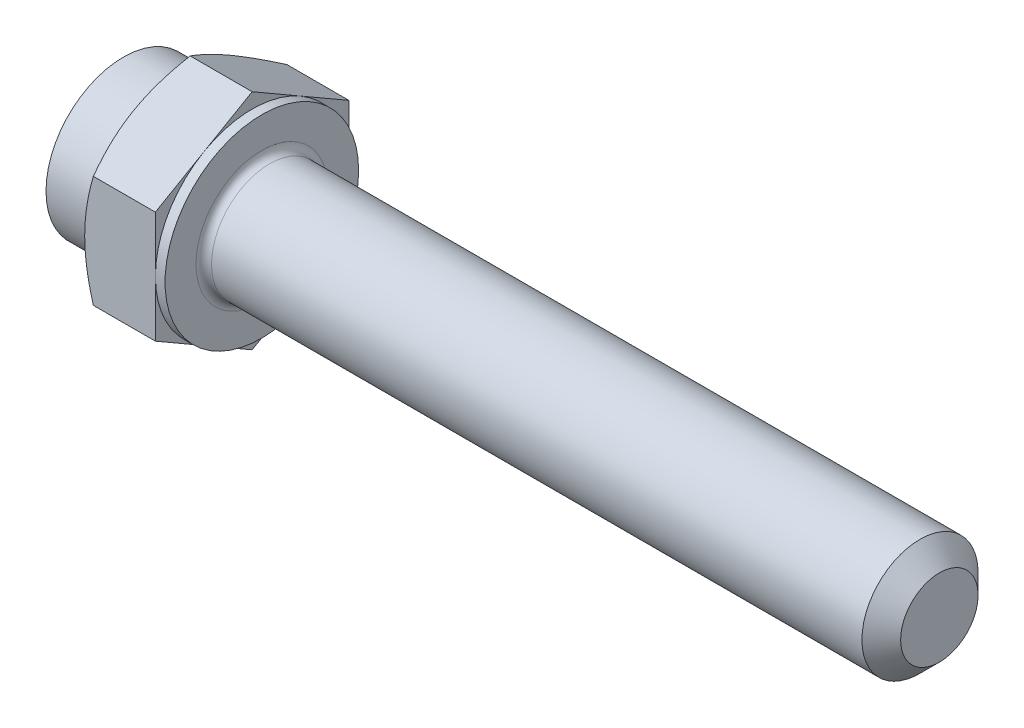
SolidWorks part; units mm, degrees
extrude "基体-拉伸" add sketch "草图1" along normal blind 4.15
sketch "草图1" plane through (0, 0, 0) normal (1, 0, 0) x (0, 0, -1)
  line L0 (5, 2.8868) -> (5, -2.8868)
  line L1 (-5, 2.8868) -> (-5, -2.8868)
  line L2 (5, -2.8868) -> (0, -5.7735)
  line L3 (0, -5.7735) -> (-5, -2.8868)
  line L4 (5, 2.8868) -> (0, 5.7735)
  line L5 (0, 5.7735) -> (-5, 2.8868)
revolve "切除-旋转1" cut sketch "草图3" angle 360 about L6
sketch "草图3" plane through (0, 0, 0) normal (0, 0, 1) x (1, 0, 0)
  line L0 (0, 5) -> (3.3333, 10.7735)
  line L1 (0, 5.7735) -> (0, 2.8868) construction
  line L2 (3.3333, 10.7735) -> (3.3333, 15.7735)
  line L3 (3.3333, 15.7735) -> (-10, 15.7735)
  line L4 (-10, 15.7735) -> (-10, 5)
  line L5 (-10, 5) -> (0, 5)
  line L6 (0, 0) -> (99.06, 0) construction
  line L7 (4.15, 5.7735) -> (0, 5.7735) construction
revolve "凸台-旋转1" add sketch "草图2" angle 360 about L7
sketch "草图2" plane through (0, 0, 0) normal (0, 0, 1) x (1, 0, 0)
  line L0 (0, 2.8868) -> (0, -2.8868) construction
  line L1 (0, 0) -> (39.15, 0)
  line L2 (0, 0) -> (0, 3)
  line L3 (0, 3) -> (39.15, 3)
  line L4 (39.15, 0) -> (39.15, 1.9175)
  line L5 (4.15, 5.7735) -> (4.15, 2.8868) construction
  line L7 (0, 0) -> (96.52, 0) construction
  line L8 (39.15, -1.9175) -> (90.335, -3) construction
  line L9 (0, -3) -> (90.335, -3) construction
  line L10 (5.4, 15.24) -> (5.4, -1.27) construction
  line L11 (9.15, 15.24) -> (9.15, -1.27) construction
  line L12 (4.15, 2.8868) -> (4.15, -2.8868) construction
  line L14 (39.15, 3) -> (39.15, 1.9175)
  dimension "l" = 35
  dimension "m" = 6
  dimension "Minor_dia" = 3.835
  dimension "p" = 1.25
  dimension "h" = 30
cosmetic thread "螺旋线1" parameters "Thread_length"=33.75, "Thread_minor"=3.835
material "不锈钢螺钉"
ref_plane "前视" through (0, 0, 0) normal (0, 0, 1) x (1, 0, 0)
ref_plane "上视" through (0, 0, 0) normal (0, 1, 0) x (1, 0, 0)
ref_plane "右视" through (0, 0, 0) normal (1, 0, 0) x (0, 0, -1)
sketch "草图5" plane through (0, 0, 0) normal (0, 0, 1) x (1, 0, 0)
  line L0 (4.15, 5) -> (0.8167, 10.7735)
  line L1 (4.15, 5.7735) -> (4.15, 2.8868) construction
  line L2 (0.8167, 10.7735) -> (0.8167, 15.7735)
  line L3 (0.8167, 15.7735) -> (10.8167, 15.7735)
  line L4 (10.8167, 15.7735) -> (10.8167, 5)
  line L5 (10.8167, 5) -> (4.15, 5)
  line L7 (4.15, 5.7735) -> (0.4466, 5.7735) construction
  line L8 (0, 0) -> (99.06, 0) construction
  line L9 (0, 0) -> (99.06, 0) construction
revolve "切除-旋转2" cut sketch "草图5" angle 360 about L8
sketch "草图4" plane through (0, 0, 0) normal (0, 0, 1) x (1, 0, 0)
  line L1 (4.15, 5.7735) -> (4.15, 2.8868) construction
  line L2 (4.15, 5) -> (3.65, 5)
  line L3 (4.15, 5) -> (4.15, 15.7735)
  line L4 (4.15, 15.7735) -> (3.65, 15.7735)
  line L5 (0, 0) -> (95.25, 0) construction
  line L6 (0, 0) -> (96.52, 0) construction
  line L7 (3.65, 5) -> (3.65, 15.7735)
  line L8 (3.7034, 5.7735) -> (0.4466, 5.7735) construction
revolve "切除-旋转3" cut sketch "草图4" angle 360 about L5
chamfer "倒角" distance 1 angle 45 1 edges at (39.15, 0, 3)
fillet "圆角" radius 0.4 1 edges at (4.15, 0, -3)
sketch "草图6" plane through (0, 0, 0) normal (0, 0, 1) x (1, 0, 0)
  line L0 (5.175, -1.9175) -> (4.55, -3)
  line L1 (5.175, -1.9175) -> (5.8, -3)
  line L2 (5.8, -3) -> (5.8, -3.75)
  line L3 (-3.175, 0) -> (5.1513, 0) construction
  line L5 (5.8, -3.75) -> (4.55, -3.75)
  line L6 (4.55, -3.75) -> (4.55, -3)
  arc A0 (4.55, -3) -> (4.15, -3.4) centre (4.55, -3.4) ccw construction
revolve "切除-旋转4" [suppressed] cut sketch "草图6" angle 360 about L3
pattern_linear "阵列(线性)1" [suppressed]
sketch "草图7" plane through (0, 0, 0) normal (-1, 0, 0) x (0, 0, 1)
  circle A0 centre (0, 0) radius 4
  dimension "D1" = 8
extrude "切除-拉伸1" cut sketch "草图7" against normal blind 3
sketch "草图8" plane through (3, 0, 0) normal (-1, 0, 0) x (0, 0, 1)
  circle A0 centre (0, 0) radius 4
  dimension "D1" = 8
extrude "凸台-拉伸1" add sketch "草图8" along normal blind 6 separate body
equation "\"D3@草图1\" = \"s@草图1\" / 2"
equation "\"D4@草图1\" = \"D3@草图1\""
equation "\"D5@草图1\" = \"D4@草图1\""
equation "\"D1@草图3\" = \"s@草图1\" / 2"
equation "\"D1@草图5\" = \"s@草图1\" / 2"
equation "\"Head_ch_ang@草图5\" = \"Head_ch_ang@草图3\""
equation "\"D1@草图4\" = \"s@草图1\""
equation "\"Diameter@草图6\" = \"m@草图2\""
equation "\"Overcut@草图6\" = \"m@草图2\" * 1.25"
equation "\"Minor_dia@草图2\" = \"m@草图2\"-\"p@草图2\" * 1.732"
equation "\"Thread_minor@螺旋线1\" = \"Minor_dia@草图2\""
equation "\"Thread_minor@草图6\" = \"Minor_dia@草图2\""
equation "\"D1@倒角\" = \"p@草图2\"*0.8"
equation "\"Thread_length@螺旋线1\" = \"l@草图2\" - \"p@草图2\""
equation "\"Num_threads@阵列(线性)1\" = \"l@草图2\" / \"p@草图2\""
